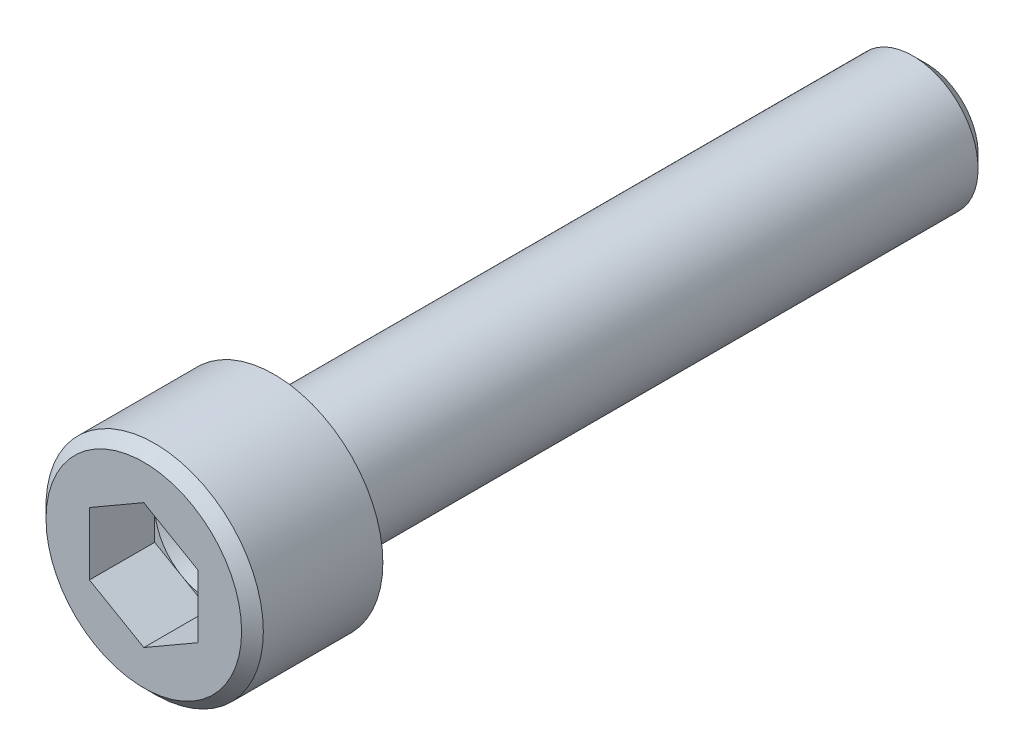
from build123d import *

# Parameters (mm, degrees)
SKETCH_1_W          = 5
SKETCH_1_H          = 6
SKETCH_2_R          = 3
EXTRUDE_1_DEPTH     = 30
CUT_EXTRUDE_1_DEPTH = 3
CHAMFER_1_SIZE      = 0.5
CHAMFER_2_SIZE      = 0.6135


with BuildPart() as part:
    # 草图1 → 旋转1 (revolve)
    with BuildSketch(Plane(origin=(0, 0, 0), x_dir=(1, 0, 0), z_dir=(0, 1, 0))):
        with Locations((2.5, -3)):
            Rectangle(SKETCH_1_W, SKETCH_1_H)
    revolve(axis=Axis((0, 0, 0), (0, 0, 1)))

    # 草图2 → 凸台-拉伸1 (add)
    with BuildSketch(Plane(origin=(0, 0, 0), x_dir=(-1, 0, 0), z_dir=(0, 0, -1))):
        Circle(SKETCH_2_R)
    extrude(amount=EXTRUDE_1_DEPTH)

    # 草图3 → 切除-拉伸1 (cut)
    with BuildSketch(Plane.XY.offset(6)):
        Polygon((2.5, 1.443375673), (0, 2.886751346), (-2.5, 1.443375673), (-2.5, -1.443375673), (0, -2.886751346), (2.5, -1.443375673), align=None)
    extrude(amount=-CUT_EXTRUDE_1_DEPTH, mode=Mode.SUBTRACT)

    # 草图4 → 切除-旋转1 (revolve, cut)
    with BuildSketch(Plane.XZ):
        Polygon((2.5, 3), (0, 3), (0, 1.556624327), align=None)
    revolve(axis=Axis((0, 0, 3), (0, 0, -1)), mode=Mode.SUBTRACT)

    # 倒角1
    chamfer_1_edges = [part.edges().sort_by_distance(p)[0] for p in [
        (-5, 0, 6),
    ]]
    chamfer(chamfer_1_edges, length=CHAMFER_1_SIZE)

    # 倒角2
    chamfer_2_edges = [part.edges().sort_by_distance(p)[0] for p in [
        (3, 0, -30),
    ]]
    chamfer(chamfer_2_edges, length=CHAMFER_2_SIZE)


solid = part.part
